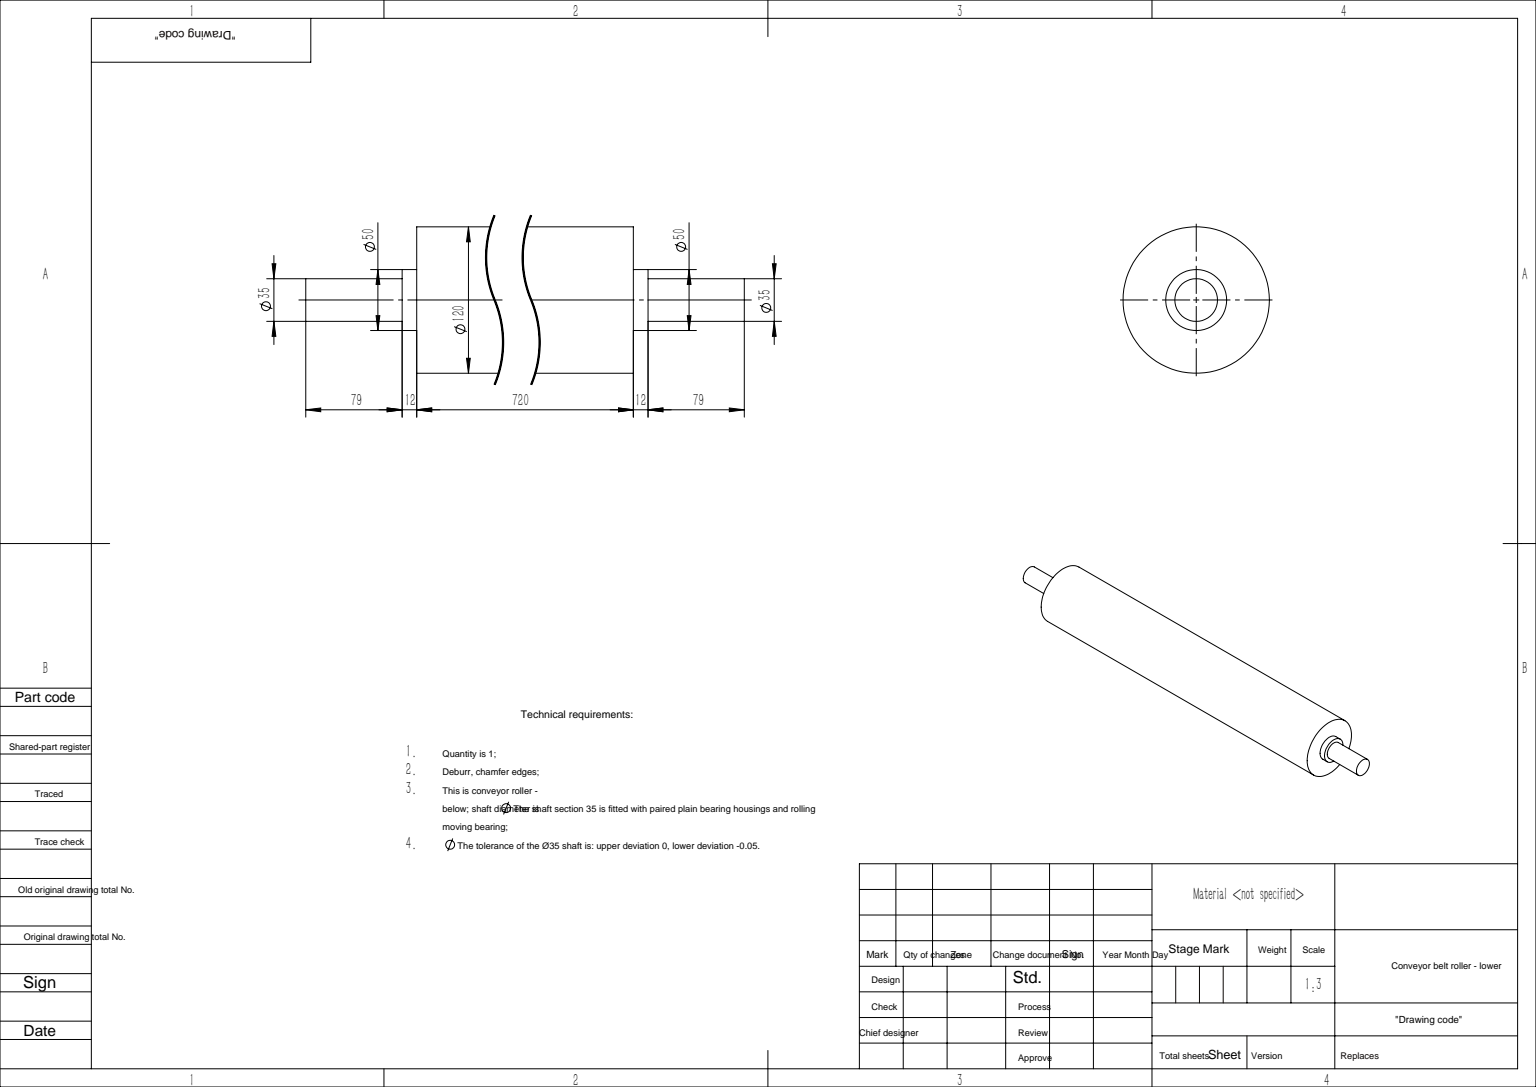
from build123d import *


with BuildPart() as part:
    # 草图1 → 旋转1 (revolve)
    with BuildSketch(Plane.XY, mode=Mode.PRIVATE) as revolve_1_sk:
        Polygon((-360, 60), (360, 60), (360, 25), (372, 25), (372, 17.5), (451, 17.5), (451, 0), (-451, 0), (-451, 17.5), (-372, 17.5), (-372, 25), (-360, 25), align=None)
    revolve(revolve_1_sk.sketch.rotate(Axis((-451, 0, 0), (1, 0, 0)), 90), axis=Axis((-451, 0, 0), (1, 0, 0)))


solid = part.part
